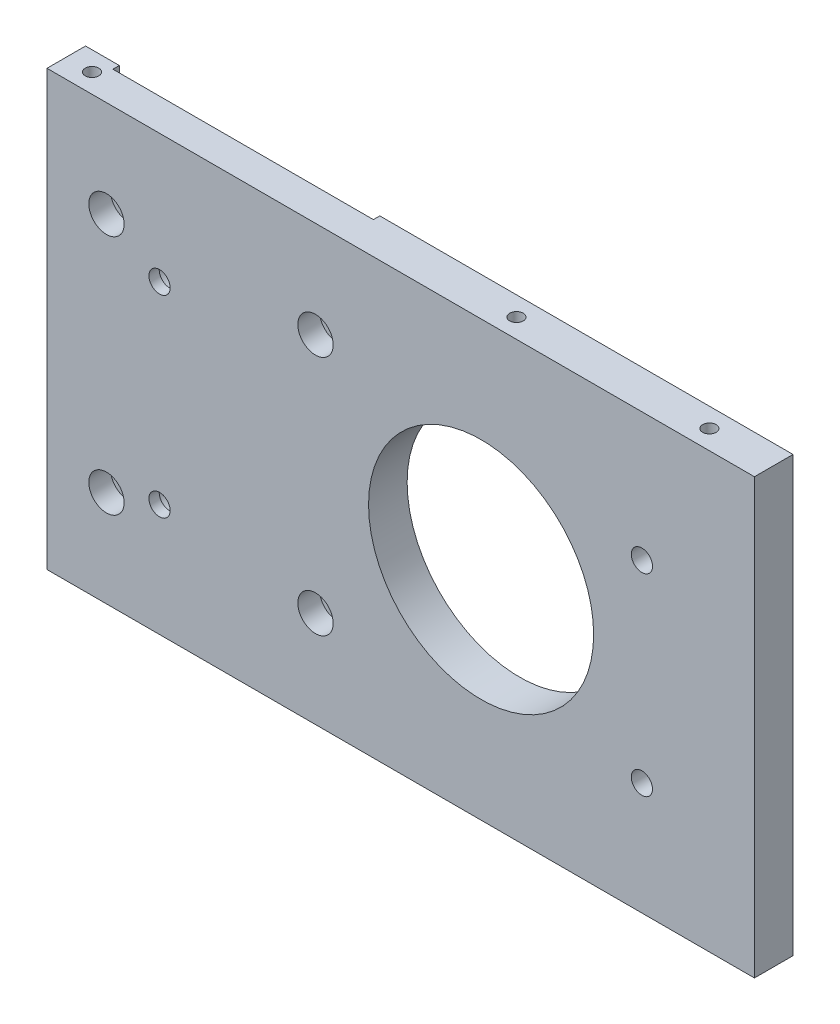
from build123d import *

# Parameters (mm, degrees)
SKETCH_1_W                      = 220
SKETCH_1_H                      = 135
EXTRUDE_1_DEPTH                 = 12
HOLE_WIZARD_1_D                 = 6.6
HOLE_WIZARD_1_CBORE_D           = 11
HOLE_WIZARD_1_CBORE_DEPTH       = 6.8
SKETCH_4_W                      = 81
SKETCH_4_H                      = 135
CUT_EXTRUDE_1_DEPTH             = 2
HOLE_WIZARD_2_D                 = 6.6
HOLE_WIZARD_2_CBORE_D           = 11
HOLE_WIZARD_2_CBORE_DEPTH       = 6.8
HOLE_WIZARD_3_D                 = 6.6
HOLE_WIZARD_3_CBORE_D           = 11
HOLE_WIZARD_3_CBORE_DEPTH       = 6.8
CUT_EXTRUDE_2_REACH             = 131.616
SKETCH_9_R                      = 35
CUT_EXTRUDE_2_DIRECTION_2_DEPTH = 130.615778361
HOLE_WIZARD_M5_1_D              = 4.2
HOLE_WIZARD_M5_1_DEPTH          = 12.4
HOLE_WIZARD_M5_1_TIP            = 1.2618073


with BuildPart() as part:
    # 草图1 → 凸台-拉伸1 (new body)
    with BuildSketch(Plane.XY):
        Rectangle(SKETCH_1_W, SKETCH_1_H)
    extrude(amount=EXTRUDE_1_DEPTH)

    # 打孔尺寸(%根据)内六角圆柱头螺钉的类型1 (through all)
    with Locations(Plane.XY.offset(12)):
        with Locations((-91.500000058, 37.5), (-26.500000058, 37.5), (-91.500000058, -37.5), (-26.500000058, -37.5)):
            CounterBoreHole(HOLE_WIZARD_1_D / 2, HOLE_WIZARD_1_CBORE_D / 2, HOLE_WIZARD_1_CBORE_DEPTH)

    # 草图4 → 切除-拉伸1 (cut)
    with BuildSketch(Plane(origin=(0, 0, 0), x_dir=(-1, 0, 0), z_dir=(0, 0, -1))):
        with Locations((59.000000058, 0)):
            Rectangle(SKETCH_4_W, SKETCH_4_H)
    extrude(amount=-CUT_EXTRUDE_1_DEPTH, mode=Mode.SUBTRACT)

    # 打孔尺寸(%根据)内六角圆柱头螺钉的类型2 (through all)
    with Locations(Plane(origin=(0, 0, 2), x_dir=(-1, 0, 0), z_dir=(0, 0, -1))):
        with Locations((75, -32.5), (75, 27.5)):
            CounterBoreHole(HOLE_WIZARD_2_D / 2, HOLE_WIZARD_2_CBORE_D / 2, HOLE_WIZARD_2_CBORE_DEPTH)

    # 打孔尺寸(%根据)内六角圆柱头螺钉的类型3 (through all)
    with Locations(Plane(origin=(0, 0, 0), x_dir=(-1, 0, 0), z_dir=(0, 0, -1))):
        with Locations((-75, -32.5), (-75, 27.5)):
            CounterBoreHole(HOLE_WIZARD_3_D / 2, HOLE_WIZARD_3_CBORE_D / 2, HOLE_WIZARD_3_CBORE_DEPTH)

    # 草图9 → 切除-拉伸2 (cut, up to next)
    with BuildSketch(Plane(origin=(0, 0, 0), x_dir=(-1, 0, 0), z_dir=(0, 0, -1)), mode=Mode.PRIVATE) as cut_extrude_2_sk1:
        with Locations(Location((-25, 0, 0), (0, 0, 180))):
            Circle(SKETCH_9_R)
    cut_extrude_2_tool1 = extrude(cut_extrude_2_sk1.sketch, amount=-CUT_EXTRUDE_2_REACH, mode=Mode.PRIVATE) & part.part
    add(cut_extrude_2_tool1.solids().sort_by_distance((25, 0, 0))[0], mode=Mode.SUBTRACT)

    # 草图9 → 切除-拉伸2 direction 2 (cut)
    with BuildSketch(Plane(origin=(0, 0, 0), x_dir=(-1, 0, 0), z_dir=(0, 0, -1))):
        with Locations(Location((-25, 0, 0), (0, 0, 180))):
            Circle(SKETCH_9_R)
    extrude(amount=CUT_EXTRUDE_2_DIRECTION_2_DEPTH, mode=Mode.SUBTRACT)

    # M5 螺纹孔1
    with Locations(Plane(origin=(0, 67.5, 0), x_dir=(1, 0, 0), z_dir=(0, 1, 0))):
        with Locations((90, -6), (30, -6), (-102, -6)):
            Hole(HOLE_WIZARD_M5_1_D / 2, depth=HOLE_WIZARD_M5_1_DEPTH)
            with Locations((0, 0, -(HOLE_WIZARD_M5_1_DEPTH + HOLE_WIZARD_M5_1_TIP / 2))):  # 118° drill point
                Cone(0, HOLE_WIZARD_M5_1_D / 2, HOLE_WIZARD_M5_1_TIP, mode=Mode.SUBTRACT)


solid = part.part
